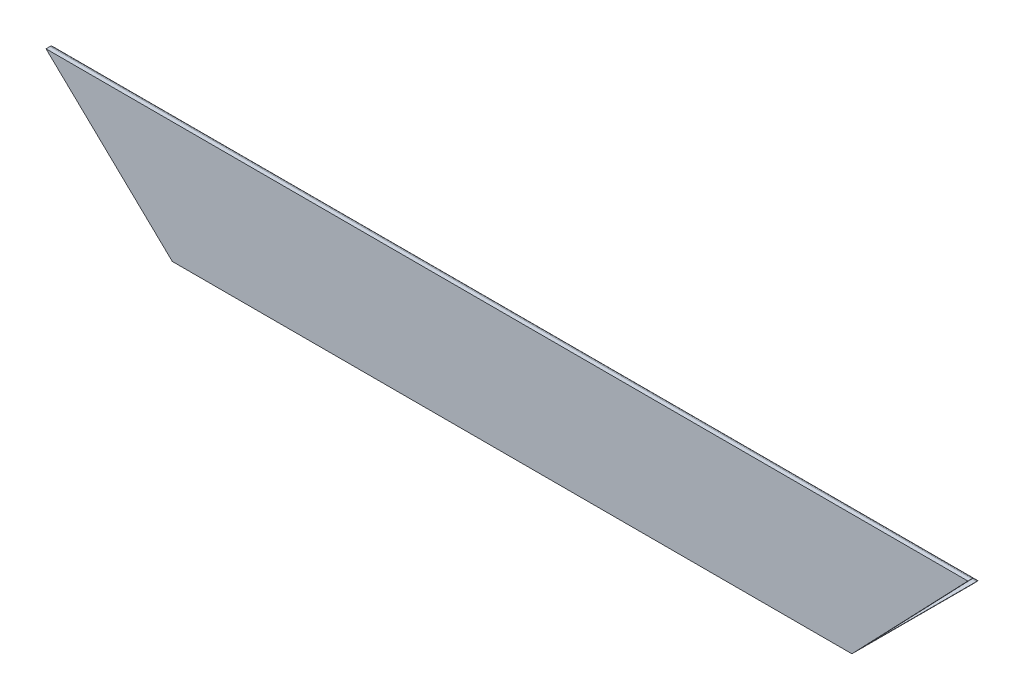
SolidWorks part; units mm, degrees
material "普通碳钢"
ref_plane "Front Plane" through (0, 0, 0) normal (0, 0, 1) x (1, 0, 0)
ref_plane "Top Plane" through (0, 0, 0) normal (0, 1, 0) x (1, 0, 0)
ref_plane "Right Plane" through (0, 0, 0) normal (1, 0, 0) x (0, 0, -1)
sketch "Sketch1" plane through (0, 0, 0) normal (1, 0, 0) x (0, 0, -1)
  line L1 (-44, 47.3) -> (-44, -32)
  line L2 (-32, -44) -> (47.3, -44)
  line L3 (50, -46.7) -> (50, -50)
  line L4 (50, -50) -> (-50, -50)
  line L5 (-50, -50) -> (-50, 50)
  line L6 (-50, 50) -> (-46.7, 50)
  arc A0 (-32, -44) -> (-44, -32) centre (-32, -32) cw
  arc A1 (-44, 47.3) -> (-46.7, 50) centre (-46.7, 47.3) ccw
  arc A2 (50, -46.7) -> (47.3, -44) centre (47.3, -46.7) ccw
  point P12 (0, -50)
  point P14 (-50, 0)
  dimension "D5" = 12
  dimension "D6" = 2.7
  dimension "D7" = 2.7
  dimension "D1" = 100
  dimension "D2" = 100
  dimension "D3" = 6
  dimension "D4" = 6
extrude "Extrude1" add sketch "Sketch1" along normal mid plane 1800
sketch "Sketch2" plane through (0, 0, 50) normal (0, 0, 1) x (1, 0, 0)
  line L0 (-900, 50) -> (-535.3959, 430.5166) construction
  line L1 (-535.3959, 430.5166) -> (-138.2724, 50) construction
  line L2 (-138.2724, 50) -> (-900, 50)
  line L5 (-900, 50) -> (-502.8764, -330.5166)
  line L6 (-502.8764, -330.5166) -> (-138.2724, 50)
  dimension "D1" = 527
  dimension "D2" = 550
extrude "Extrude5" cut sketch "Sketch2" against normal blind 100 flip side to cut
